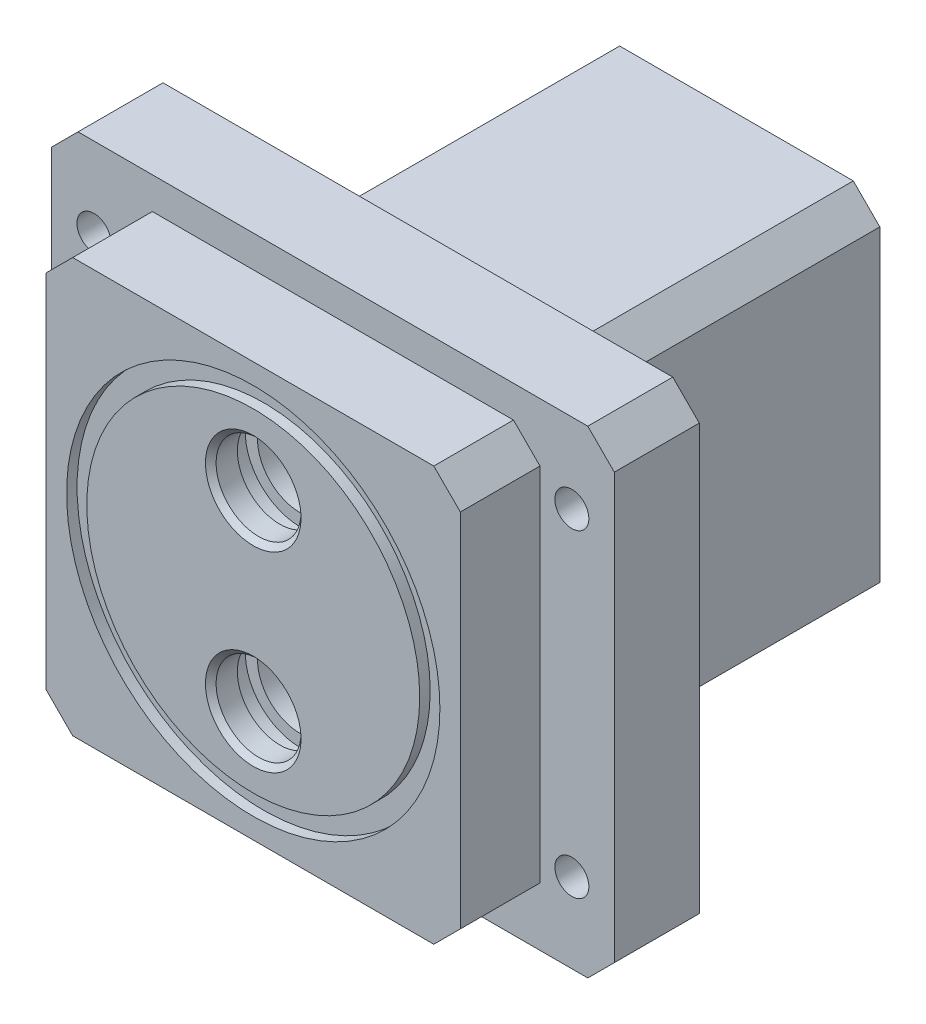
from build123d import *

# Parameters (mm, degrees)
SKETCH1_W             = 54
SKETCH1_H             = 68
BOSS_EXTRUDE1_DEPTH   = 60
SKETCH2_W             = 106
SKETCH2_H             = 90
BOSS_EXTRUDE2_DEPTH   = 16
SKETCH3_W             = 78
SKETCH3_H             = 78
BOSS_EXTRUDE3_DEPTH   = 15
CHAMFER1_SIZE         = 5
SKETCH4_R             = 35.15
SKETCH4_R_2           = 31.35
CUT_EXTRUDE1_DEPTH    = 1.97
HOLE1_D               = 16
HOLE2_D               = 22
HOLE2_DEPTH           = 63
CHAMFER2_SIZE         = 1
M5_TAPPED_HOLE1_D     = 4.2
M5_TAPPED_HOLE1_DEPTH = 10
M5_TAPPED_HOLE1_TIP   = 1.2618073
HOLE3_D               = 6.4
HOLE3_CBORE_D         = 11
HOLE3_CBORE_DEPTH     = 9
SKETCH16_R            = 10.3
CUT_EXTRUDE2_DEPTH    = 3.8


with BuildPart() as part:
    # Sketch1 → Boss-Extrude1 (new body)
    with BuildSketch(Plane.XY):
        Rectangle(SKETCH1_W, SKETCH1_H)
    extrude(amount=BOSS_EXTRUDE1_DEPTH)

    # Sketch2 → Boss-Extrude2 (add)
    with BuildSketch(Plane.XY.offset(60)):
        Rectangle(SKETCH2_W, SKETCH2_H)
    extrude(amount=BOSS_EXTRUDE2_DEPTH)

    # Sketch3 → Boss-Extrude3 (add)
    with BuildSketch(Plane.XY.offset(76)):
        Rectangle(SKETCH3_W, SKETCH3_H)
    extrude(amount=BOSS_EXTRUDE3_DEPTH)

    # Chamfer1
    chamfer1_edges = [part.edges().sort_by_distance(p)[0] for p in [
        (-53, 45, 68),
        (-53, -45, 68),
        (53, -45, 68),
        (53, 45, 68),
        (-39, 39, 83.5),
        (-39, -39, 83.5),
        (39, -39, 83.5),
        (39, 39, 83.5),
        (27, -34, 30),
        (-27, -34, 30),
        (-27, 34, 30),
        (27, 34, 30),
    ]]
    chamfer(chamfer1_edges, length=CHAMFER1_SIZE)

    # Sketch4 → Cut-Extrude1 (cut)
    with BuildSketch(Plane.XY.offset(91)):
        Circle(SKETCH4_R)
        Circle(SKETCH4_R_2, mode=Mode.SUBTRACT)
    extrude(amount=-CUT_EXTRUDE1_DEPTH, mode=Mode.SUBTRACT)

    # Hole1 (through all)
    with Locations(Plane.XY.offset(91)):
        with Locations((0, -18), (0, 18)):
            Hole(HOLE1_D / 2)

    # Hole2
    with Locations(Plane(origin=(0, 0, 0), x_dir=(-1, 0, 0), z_dir=(0, 0, -1))):
        with Locations((0, 18), (0, -18)):
            Hole(HOLE2_D / 2, depth=HOLE2_DEPTH)

    # Chamfer2
    chamfer2_edges = [part.edges().sort_by_distance(p)[0] for p in [
        (8, 18, 91),
        (8, -18, 91),
        (-11, -18, 0),
        (-11, 18, 0),
    ]]
    chamfer(chamfer2_edges, length=CHAMFER2_SIZE)

    # M5 Tapped Hole1
    with Locations(Plane(origin=(0, 0, 0), x_dir=(-1, 0, 0), z_dir=(0, 0, -1))):
        with Locations((20, -18), (20, 18), (-20, 18), (-20, -18)):
            Hole(M5_TAPPED_HOLE1_D / 2, depth=M5_TAPPED_HOLE1_DEPTH)
            with Locations((0, 0, -(M5_TAPPED_HOLE1_DEPTH + M5_TAPPED_HOLE1_TIP / 2))):  # 118° drill point
                Cone(0, M5_TAPPED_HOLE1_D / 2, M5_TAPPED_HOLE1_TIP, mode=Mode.SUBTRACT)

    # Hole3 (through all)
    with Locations(Plane(origin=(0, 0, 60), x_dir=(-1, 0, 0), z_dir=(0, 0, -1))):
        with Locations((45, -30), (45, 30), (-45, 30), (-45, -30)):
            CounterBoreHole(HOLE3_D / 2, HOLE3_CBORE_D / 2, HOLE3_CBORE_DEPTH)

    # Sketch16 → Cut-Extrude2 (cut)
    with BuildSketch(Plane.XY.offset(86)):
        with Locations((0, 18)):
            Circle(SKETCH16_R)
        with Locations((0, -18)):
            Circle(SKETCH16_R)
    extrude(amount=-CUT_EXTRUDE2_DEPTH, mode=Mode.SUBTRACT)


solid = part.part
